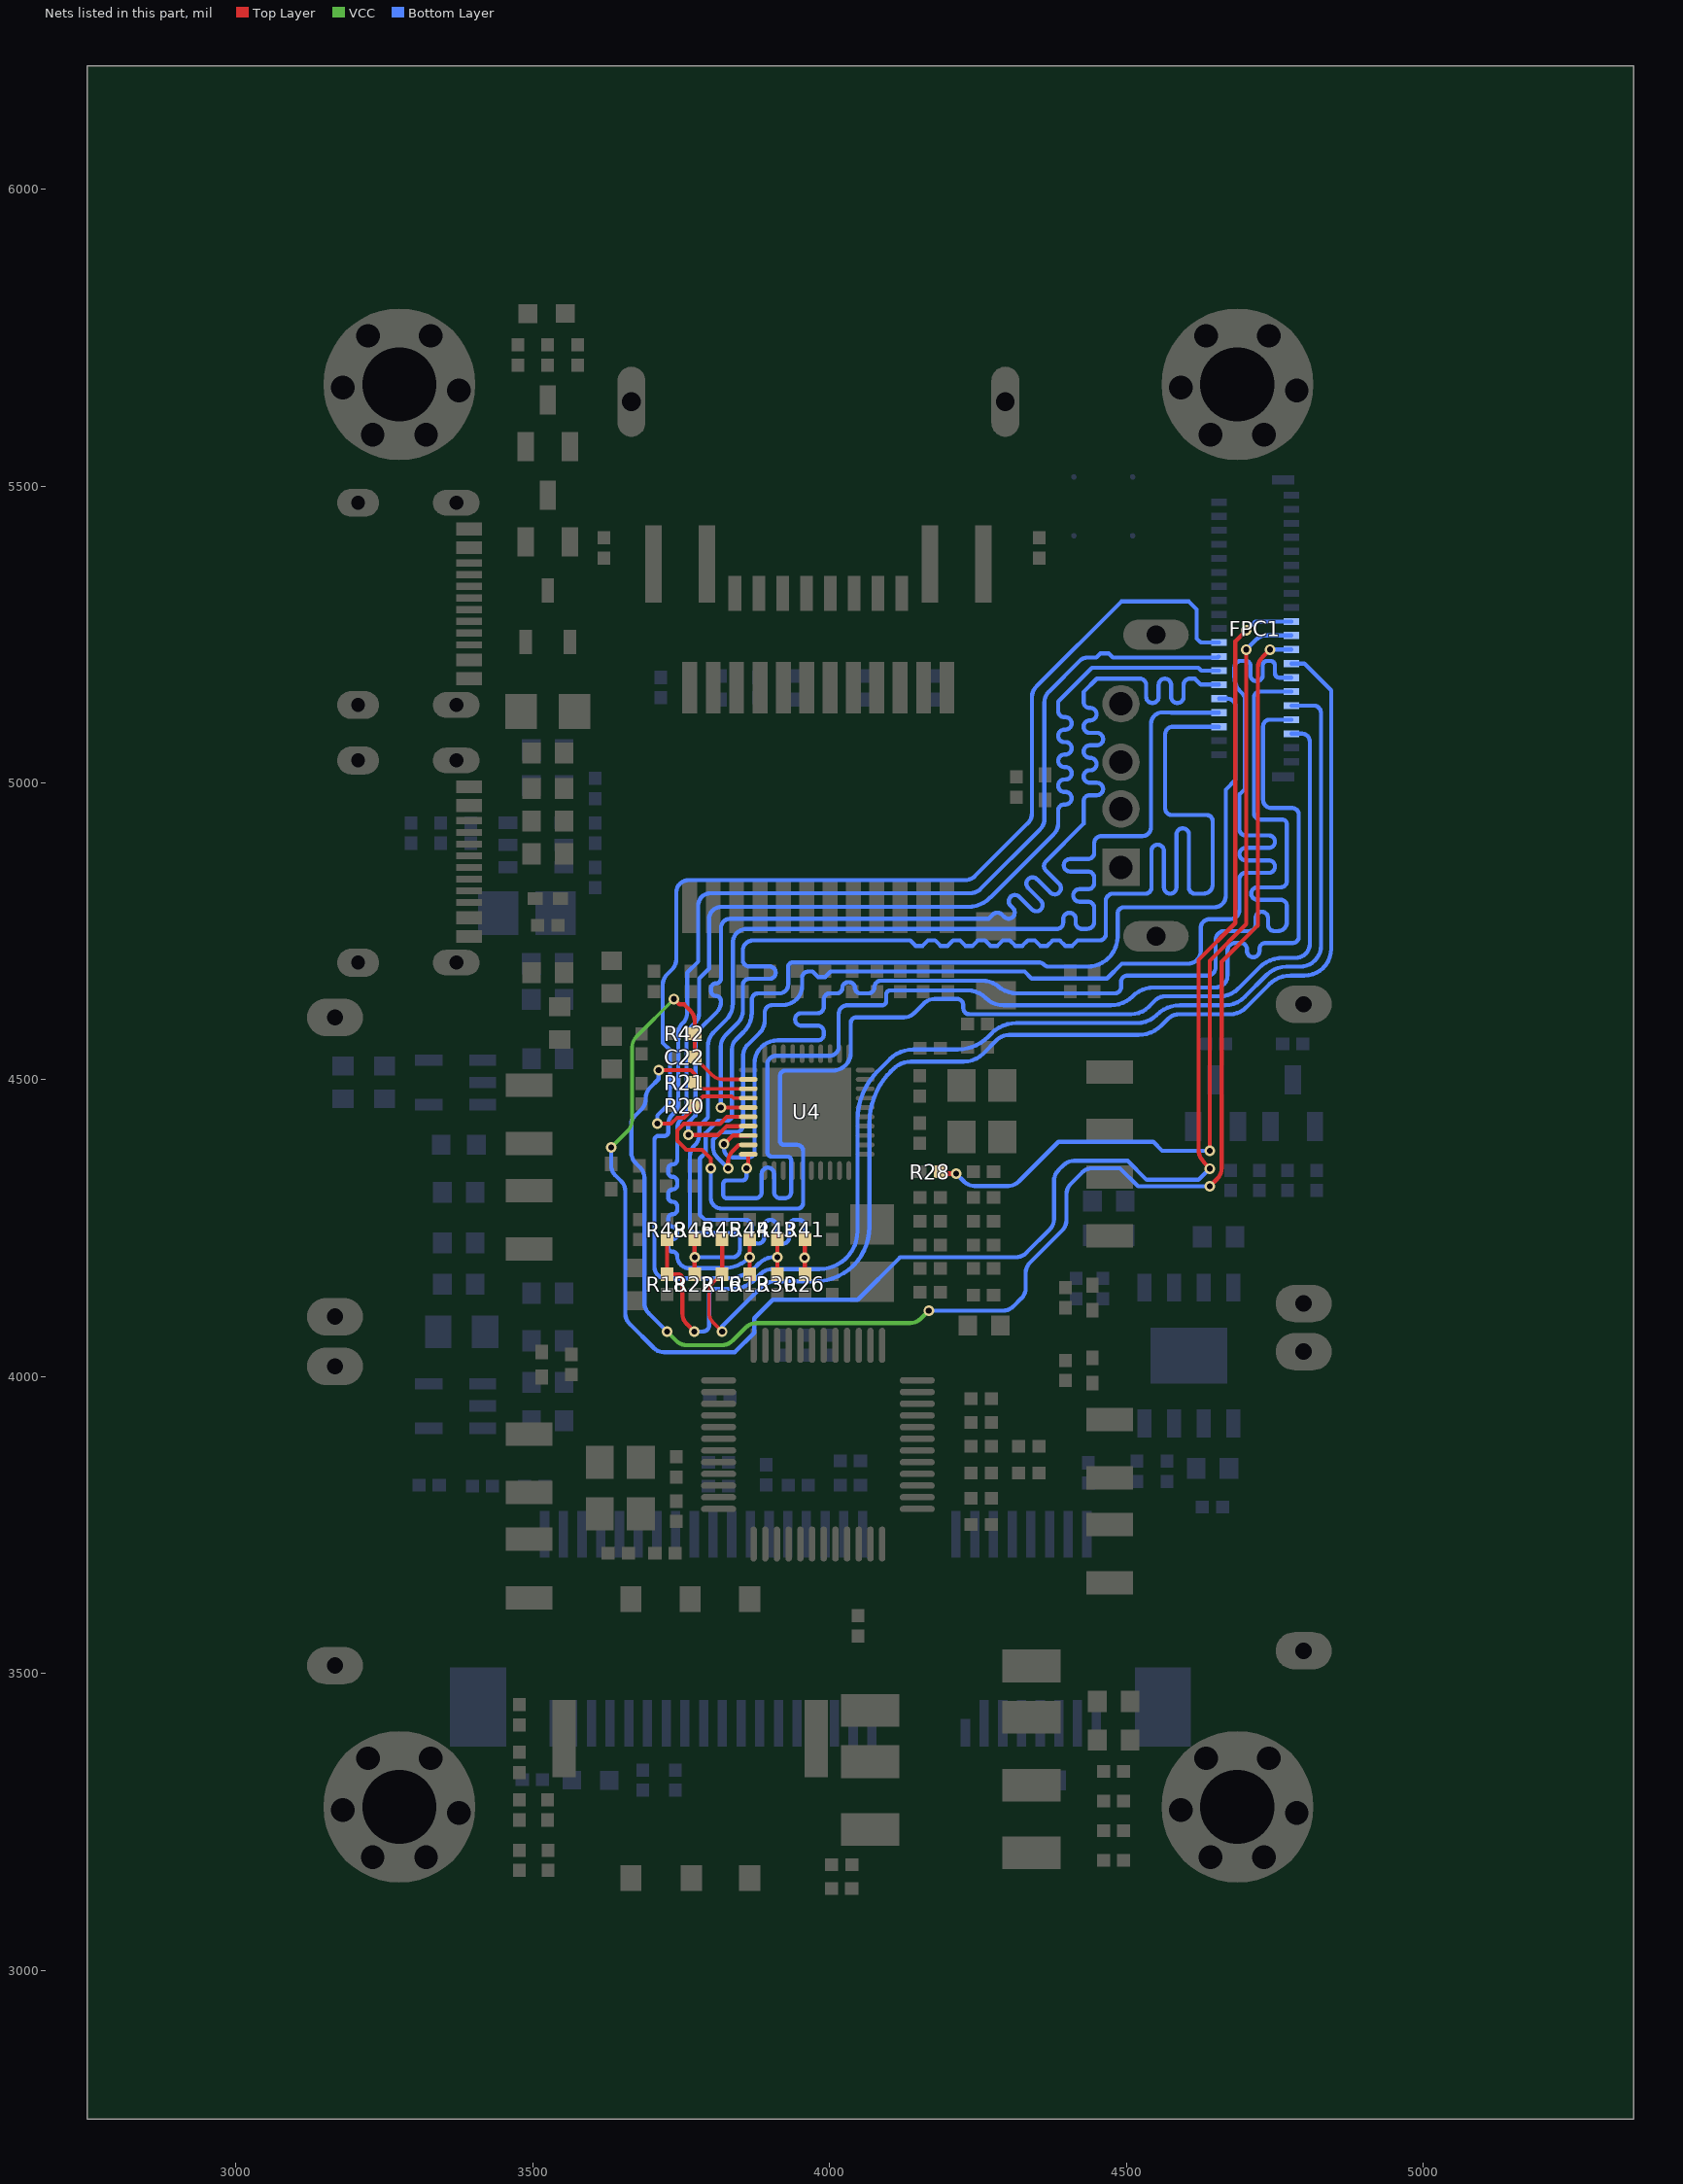
[diagram p0: the nets of this part, all layers, seen from the top]
# Altium PCB MISC84334.PcbDoc (part 5 of 8)
Units mil, origin at the board's own origin, x right, y up, seen from the top; angles counter-clockwise.
Board outline 2605.13 x 3457.4 mil, 4 copper layers (Top Layer, GND, VCC, Bottom Layer), stack 62.447 mil thick; 209 components, 149 nets, 735 pads, 529 vias.

## Via types
v1: diameter 18, hole 10, Top Layer to Bottom Layer, 529 vias

## Nets (pads, with @x,y where several pads share a name; then routed paths per layer and width w, separated by ;. In a path a pad name is that pad's centre, name@x,y a point inside that pad or via, vN(x,y) a via of type N, cw(c..) or ccw(c..) an arc to the next point about the centre after c; other vN are vias at no path point) (continued)
GMAC0_MCLKINOUT: FPC1.19 R28.2 | length 1451.4
  Top Layer w7: v1(4640.59,4380.59) 4640.59,4700.59 4702.29,4762.29 v1(4702.29,5224.65)
  Top Layer w8: R28.2@4186.94,4342.09 v1(4213.29,4342.09)
  Bottom Layer w7: v1@4213.39,4342.09 4226.97,4328.51 ccw(c4244.65,4346.19) 4244.65,4321.19 4301.05,4321.19 ccw(c4301.05,4346.19) 4318.73,4328.51 4385.8,4395.59 4545.59,4395.59 4560.59,4380.59 v1(4640.59,4380.59) ; v1(4702.29,5224.65) 4718.6,5240.96 cw(c4736.28,5223.28) 4736.28,5248.28 FPC1.19@4778.31,5248.27
GMAC0_MDC: FPC1.17 R21.2 U4.13 | length 2745
  Top Layer w6: R21.2@3773.13,4495.59 3783.73,4484.99 U4.13@3863.36,4484.99
  Top Layer w7: v1(3712.29,4516.19) 3766.66,4516.19 3773.13,4509.72 R21.2@3773.13,4495.59 ; v1(4640.59,4320.59) 4653.47,4333.47 ccw(c4635.79,4351.15) 4660.79,4351.15 4660.79,4698.96 4721.83,4760 4721.83,5193.84 cw(c4746.83,5193.84) 4729.16,5211.52 v1(4742.29,5224.65)
  VCC w7: v1(3726.29,4076.19) 3741.97,4060.51 ccw(c3759.65,4078.19) 3759.65,4053.19 3818.94,4053.19 ccw(c3818.94,4078.19) 3836.61,4060.51 3859.12,4083.02 cw(c3876.8,4065.34) 3876.8,4090.34 4136.09,4090.34 ccw(c4136.09,4115.34) 4153.77,4097.67 v1(4167.29,4111.19)
  Bottom Layer w7: 3689.29,4145.19 3688.29,4146.19 ; v1(3712.29,4516.19) 3712.29,4501.19 3697.91,4486.81 ccw(c3715.59,4469.14) 3690.59,4469.14 3690.59,4467.71 cw(c3665.59,4467.71) 3683.27,4450.03 3670.34,4437.1 ccw(c3680.1,4427.33) 3666.29,4427.33 3666.29,4377.55 ccw(c3691.29,4377.55) 3673.61,4359.87 3680.97,4352.51 cw(c3663.29,4334.84) 3688.29,4334.84 3688.29,4146.19 ; v1(3726.29,4076.19) 3695.61,4106.87 cw(c3713.29,4124.55) 3688.29,4124.55 3688.29,4146.19 ; v1(4167.29,4111.19) 4292.2,4111.19 ccw(c4292.2,4136.19) 4309.88,4118.51 4323.38,4132.02 ccw(c4305.71,4149.7) 4330.71,4149.7 4330.71,4174.5 cw(c4355.71,4174.5) 4338.03,4192.18 4391.97,4246.12 ccw(c4374.29,4263.8) 4399.29,4263.8 4399.29,4307.16 cw(c4424.29,4307.16) 4406.61,4324.84 4425.65,4343.87 cw(c4443.32,4326.19) 4443.32,4351.19 4489.45,4351.19 4520.05,4320.59 v1(4640.59,4320.59) ; v1(4742.29,5224.65) FPC1.17@4778.31,5224.65
GMAC0_MDIO: FPC1.18 R20.2 U4.14 | length 1887.1
  Top Layer w6: v1(3710.29,4426.19) 3733.29,4426.19 3743.29,4436.19 3755.29,4436.19 3773.13,4454.03 R20.2@3773.13,4456.33 3773.13,4458.16 3787.03,4472.05 3835.63,4472.05 3838.49,4469.19 U4.14@3863.36,4469.19
  Bottom Layer w7: v1@3711.29,4426.19 v1(3710.29,4426.19) 3710.29,4439.99 3723.97,4453.67 ccw(c3706.29,4471.34) 3731.29,4471.34 3731.29,4550.19 3719.29,4562.19 3719.29,4659.84 cw(c3744.29,4659.84) 3726.61,4677.51 3734.72,4685.62 ccw(c3717.05,4703.3) 3742.05,4703.3 3742.05,4815.59 cw(c3762.65,4815.59) 3762.65,4836.19 4227.94,4836.19 ccw(c4227.94,4861.19) 4245.61,4843.51 4333.97,4931.87 ccw(c4316.29,4949.55) 4341.29,4949.55 4341.29,5144.84 cw(c4366.29,5144.84) 4348.61,5162.51 4491.69,5305.59 4605.59,5305.59 4618.84,5292.34 4618.84,5243.21 4625.59,5236.46 FPC1.18@4656.27,5236.46
GMAC0_RSTN: C22.2 FPC1.21 R42.1 U4.12 | length 3058.2
  Top Layer w6: R42.1@3773.13,4578.09 C22.2@3773.13,4538.09 3773.13,4537.35 3802.47,4508.01 ccw(c3820.15,4525.69) 3820.15,4500.69 U4.12@3863.36,4500.69
  Top Layer w7: v1(3738.29,4636.19) 3747.39,4627.09 3755.39,4627.09 3765.81,4616.67 cw(c3748.13,4599) 3773.13,4599 R42.1@3773.13,4578.09 ; v1(4640.59,4350.59) 4628.53,4364.26 cw(c4647.86,4381.31) 4622.09,4381.31 4622.09,4702.09 4683.79,4763.79 4683.79,5238.4 v1(4702.29,5256.9)
  VCC w6: v1(3632.29,4386.19) 3660.27,4414.17 ccw(c3642.59,4431.85) 3667.59,4431.85 3667.59,4555.14 cw(c3692.59,4555.14) 3674.91,4572.81 v1(3738.29,4636.19)
  Bottom Layer w7: v1(3632.29,4386.19) 3632.29,4356.55 ccw(c3657.29,4356.55) 3639.61,4338.87 3648.97,4329.51 cw(c3631.29,4311.84) 3656.29,4311.84 3656.29,4106.55 ccw(c3681.29,4106.55) 3663.61,4088.87 3703.97,4048.51 ccw(c3721.65,4066.19) 3721.65,4041.19 3840.58,4041.19 3873.48,4074.09 3873.48,4098.6 3904.57,4129.69 4047.7,4129.69 4119.2,4201.19 4313.94,4201.19 ccw(c4313.94,4226.19) 4331.61,4208.51 4370.97,4247.87 ccw(c4353.29,4265.55) 4378.29,4265.55 4378.29,4329.81 cw(c4403.29,4329.81) 4385.61,4347.49 4394.49,4356.37 cw(c4412.17,4338.69) 4412.17,4363.69 4502.49,4363.69 4534.59,4331.59 4621.59,4331.59 v1(4640.59,4350.59) ; v1(4702.29,5256.9) 4717.29,5271.9 FPC1.21@4778.31,5271.89
GMAC0_RXCLK: FPC1.10 R26.2 R41.2 | length 2122.7
  Top Layer w7: R26.2@3958.66,4172.63 R41.2@3958.66,4230.81
  Bottom Layer w7: v1(3958.29,4200.19) 3958.29,4255.19 ccw(c3949.29,4255.19) 3949.29,4264.19 3942.71,4264.19 ccw(c3942.71,4253.69) 3932.21,4253.69 3932.21,4234.59 cw(c3921.71,4234.59) 3911.21,4234.59 3911.21,4253.69 ccw(c3900.71,4253.69) 3890.21,4253.69 3890.21,4234.59 cw(c3879.71,4234.59) 3869.21,4234.59 3869.21,4253.69 ccw(c3858.71,4253.69) 3858.71,4264.19 3790.29,4264.19 3781.8,4272.68 3781.8,4367.85 3791.79,4377.84 3791.79,4410.71 3812.29,4431.19 3827.29,4431.19 ccw(c3827.29,4439.69) 3835.79,4439.69 3835.79,4551.48 cw(c3858.27,4551.48) 3842.37,4567.37 3855.59,4580.59 ccw(c3822.52,4613.67) 3869.29,4613.67 3869.29,4635.08 cw(c3879.8,4635.08) 3879.8,4645.59 3915.59,4645.59 ccw(c3915.59,4660.59) 3930.59,4660.59 3930.59,4690.47 cw(c3937.81,4690.47) 3937.81,4697.69 4352.74,4697.69 cw(c4352.74,4685.57) 4361.31,4694.14 ccw(c4369.88,4702.71) 4369.88,4690.59 4434.44,4690.59 ccw(c4434.44,4741.65) 4470.55,4705.55 ccw(c4434.44,4741.65) 4485.5,4741.65 4485.5,4779.75 cw(c4496.34,4779.75) 4496.34,4790.59 4648.37,4790.59 ccw(c4648.37,4809.87) 4667.65,4809.87 4667.65,4988.76 4684.29,5005.4 4684.29,5127.96 ccw(c4670.27,5127.96) 4680.18,5137.87 ccw(c4670.27,5127.96) 4670.27,5141.98 FPC1.10@4656.27,5141.97
GMAC0_RXD0: FPC1.14 R13.2 R44.2 | length 2125.2
  Top Layer w7: R13.2@3865.8,4172.63 v1(3865.8,4201.17) R44.2@3865.8,4230.81
  Bottom Layer w7: v1(3865.8,4201.17) cw(c3821.19,4245.79) 3821.19,4182.69 3763.93,4182.69 cw(c3763.93,4203.03) 3743.59,4203.03 ccw(c3735.99,4203.03) 3735.99,4210.63 cw(c3735.99,4218.23) 3728.39,4218.23 3728.39,4224.03 cw(c3735.99,4224.03) 3735.99,4231.63 ccw(c3735.99,4239.23) 3743.59,4239.23 3743.59,4245.03 ccw(c3735.99,4245.03) 3735.99,4252.63 cw(c3735.99,4260.23) 3728.39,4260.23 3728.39,4266.03 cw(c3735.99,4266.03) 3735.99,4273.63 ccw(c3735.99,4281.23) 3743.59,4281.23 3743.59,4287.03 ccw(c3735.99,4287.03) 3735.99,4294.63 cw(c3735.99,4302.23) 3728.39,4302.23 3728.39,4308.03 cw(c3735.99,4308.03) 3735.99,4315.63 ccw(c3735.99,4323.23) 3743.59,4323.23 3743.59,4329.03 ccw(c3735.99,4329.03) 3735.99,4336.63 cw(c3735.99,4344.23) 3728.39,4344.23 3728.39,4350.03 cw(c3735.99,4350.03) 3735.99,4357.63 ccw(c3735.99,4365.23) 3743.59,4365.23 3743.59,4417.14 cw(c3768.59,4417.14) 3750.91,4434.81 3751.97,4435.87 ccw(c3734.29,4453.55) 3759.29,4453.55 3759.29,4571.08 cw(c3784.29,4571.08) 3766.61,4588.76 3773.29,4595.44 ccw(c3755.68,4613.06) 3780.59,4613.06 3780.59,4670.59 3797.29,4687.29 3797.29,4770.84 cw(c3817.65,4770.84) 3817.65,4791.19 4232.9,4791.19 ccw(c4232.9,4845.33) 4271.18,4807.05 4377.97,4913.84 ccw(c4360.29,4931.51) 4385.29,4931.51 4385.29,4953.33 cw(c4395.79,4953.33) 4395.79,4963.83 4397.61,4963.83 ccw(c4397.61,4974.33) 4397.61,4984.83 4395.79,4984.83 cw(c4395.79,4995.33) 4395.79,5005.83 4397.61,5005.83 ccw(c4397.61,5016.33) 4397.61,5026.83 4395.79,5026.83 cw(c4395.79,5037.33) 4395.79,5047.83 4397.61,5047.83 ccw(c4397.61,5058.33) 4397.61,5068.83 4395.79,5068.83 cw(c4395.79,5079.33) 4395.79,5089.83 4397.61,5089.83 ccw(c4397.61,5100.33) 4397.61,5110.83 4395.79,5110.83 cw(c4395.79,5121.33) 4385.29,5121.33 4385.29,5137.19 4442.24,5194.14 4621.44,5194.14 4626.36,5189.22 FPC1.14@4656.27,5189.22
GMAC0_RXD1: FPC1.15 R16.2 R45.2 | length 2125.3
  Top Layer w6: v1(3819.38,4076.19) 3804.61,4090.95 cw(c3822.29,4108.63) 3797.29,4108.63 3797.29,4141.59 cw(c3822.29,4141.59) 3804.61,4159.27 3817.98,4172.63 R16.2@3819.38,4172.63
  Top Layer w7: R16.2@3819.38,4172.63 R45.2@3819.38,4230.81
  Bottom Layer w7: v1(3819.38,4076.19) 3819.38,4085.03 3885.76,4151.41 cw(c3907.92,4129.26) 3907.92,4160.59 3975.88,4160.59 ccw(c3975.88,4252.01) 4067.29,4252.01 4067.29,4426.65 cw(c4192.12,4426.65) 4097.07,4507.56 4102.78,4513.28 cw(c4118.29,4503.19) 4108.2,4518.7 cw(c4136.91,4489.98) 4115.77,4524.65 cw(c4136.91,4489.98) 4136.91,4530.59 4226.3,4530.59 ccw(c4226.3,4577.16) 4259.23,4544.23 4282.44,4567.44 cw(c4302.12,4547.75) 4302.12,4575.59 4520.6,4575.59 ccw(c4520.6,4630.46) 4559.4,4591.66 4570.54,4602.8 cw(c4589.35,4583.98) 4589.35,4610.59 4675.41,4610.59 ccw(c4675.41,4647.24) 4701.32,4621.32 4740.59,4660.59 cw(c4776.8,4624.38) 4776.8,4675.59 4800.09,4675.59 ccw(c4800.09,4720.78) 4845.28,4720.78 4845.28,5155.9 4800.15,5201.03 FPC1.15@4778.31,5201.03
GMAC0_RXD2: FPC1.8 R22.2 R46.2 | length 2122.7
  Top Layer w7: R22.2@3772.95,4172.63 R46.2@3772.95,4230.81
  Bottom Layer w7: v1(3773.29,4201.19) 3836.29,4201.19 ccw(c3836.29,4214.19) 3849.29,4214.19 3849.29,4234.18 ccw(c3841.28,4234.18) 3841.28,4242.19 3775.16,4242.19 cw(c3775.16,4252.42) 3764.93,4252.42 3764.93,4371.25 cw(c3789.93,4371.25) 3772.25,4388.93 3773.47,4390.14 ccw(c3755.79,4407.82) 3780.79,4407.82 3780.79,4421.95 3795.29,4436.45 3795.29,4556.63 cw(c3828.26,4556.63) 3804.95,4579.95 3825.59,4600.59 ccw(c3797.34,4628.84) 3837.29,4628.84 3837.29,4730.84 cw(c3860.65,4730.84) 3860.65,4754.19 4383.37,4754.19 ccw(c4383.37,4764.69) 4393.87,4764.69 4393.87,4770.86 cw(c4404.37,4770.86) 4414.87,4770.86 4414.87,4764.69 ccw(c4425.37,4764.69) 4425.37,4754.19 4434.19,4754.19 ccw(c4434.19,4766.09) 4446.09,4766.09 4446.09,4789.54 ccw(c4435.59,4789.54) 4435.59,4800.04 4421.09,4800.04 cw(c4421.09,4810.54) 4421.09,4821.04 4435.59,4821.04 ccw(c4435.59,4831.54) 4446.09,4831.54 4446.09,4840.38 ccw(c4435.59,4840.38) 4435.59,4850.88 4405.29,4850.88 cw(c4405.29,4861.38) 4405.29,4871.88 4435.59,4871.88 ccw(c4435.59,4882.38) 4446.09,4882.38 4446.09,4898.59 cw(c4458.09,4898.59) 4458.09,4910.59 4527.28,4910.59 ccw(c4527.28,4925.01) 4541.7,4925.01 4541.7,5099.48 cw(c4561.02,5099.48) 4561.02,5118.8 4592.83,5118.35 ; 4575.62,5118.35 4592.84,5118.35 ; FPC1.8@4656.27,5118.35 4592.84,5118.35
GMAC0_RXD3: FPC1.9 R18.2 R48.2 | length 2120
  Top Layer w7: R48.2@3726.52,4230.81 R18.2@3726.52,4172.63 3744.8,4172.63 cw(c3744.8,4165.14) 3752.29,4165.14 3752.29,4106.55 ccw(c3777.29,4106.55) 3759.61,4088.87 v1(3772.29,4076.19)
  Bottom Layer w7: v1(3772.29,4076.19) 3787.29,4076.19 ccw(c3787.29,4086.19) 3797.29,4086.19 3797.29,4137.79 cw(c3807.59,4137.79) 3807.59,4148.09 3835.59,4148.09 ccw(c3835.59,4205.07) 3875.88,4164.78 3884.97,4173.87 cw(c3902.65,4156.19) 3902.65,4181.19 3983.06,4181.19 ccw(c3983.06,4245.42) 4013.57,4188.9 ccw(c3983.06,4245.42) 4047.29,4245.42 4047.29,4432.02 cw(c4164.38,4432.02) 4081.59,4514.82 4101.28,4534.51 cw(c4141.55,4494.25) 4141.55,4551.19 4216.09,4551.19 ccw(c4216.09,4623.86) 4267.48,4572.48 4273.62,4578.62 cw(c4314.59,4537.65) 4314.59,4595.59 4517.91,4595.59 ccw(c4517.91,4643.17) 4551.56,4609.53 cw(c4590.34,4570.75) 4590.34,4625.59 4666.52,4625.59 ccw(c4666.52,4671.64) 4699.08,4639.08 4737.04,4677.04 cw(c4769.75,4644.33) 4769.75,4690.59 4792.99,4690.59 ccw(c4792.99,4725.68) 4828.08,4725.68 4828.08,5118.14 ccw(c4816.05,5118.14) 4816.05,5130.17 FPC1.9@4778.31,5130.16
GMAC0_RXDV_CRS: FPC1.16 R30.2 R43.2 | length 2122.3
  Top Layer w7: R30.2@3912.23,4172.63 v1(3912.23,4201.17) R43.2@3912.23,4230.81
  Bottom Layer w7: FPC1.16@4656.27,5212.84 cw(c4652.21,5216.9) 4652.21,5211.16 4477.56,5211.16 4470.56,5218.16 4456.56,5218.16 4449.56,5211.16 4434.14,5211.16 ccw(c4434.14,5194.55) 4422.39,5206.29 4369.61,5153.51 ccw(c4387.29,5135.84) 4362.29,5135.84 4362.29,4939.55 cw(c4337.29,4939.55) 4354.97,4921.87 4254.61,4821.51 cw(c4236.94,4839.19) 4236.94,4814.19 3799.34,4814.19 ccw(c3799.34,4793.9) 3779.05,4793.9 3779.05,4699.05 3760.59,4680.59 3760.59,4614.34 cw(c3733.35,4614.34) 3752.61,4595.09 ccw(c3770.29,4577.41) 3745.29,4577.41 3745.29,4461.55 cw(c3720.29,4461.55) 3737.97,4443.87 3734.36,4440.26 ccw(c3747.83,4426.79) 3728.78,4426.79 cw(c3710.29,4426.19) 3728.78,4425.59 3728.78,4412.41 cw(c3721.96,4412.41) 3721.96,4405.59 3712.37,4405.59 ccw(c3712.37,4398.52) 3705.29,4398.52 3705.29,4184.68 ccw(c3724.41,4184.68) 3724.41,4165.55 3826.26,4165.55 ccw(c3826.26,4238.19) 3849.97,4169.53 ccw(c3826.26,4238.19) 3854.79,4171.39 ccw(c3826.26,4238.19) 3877.62,4186.83 3881.75,4190.95 cw(c3907.26,4165.44) 3902.28,4201.17 ; 3902.28,4201.17 v1(3912.23,4201.17) ccw(c3907.26,4165.44) 3902.28,4201.17
GMAC0_TXCLK: FPC1.7 U4.20 | length 2125.1
  Top Layer w7: v1(3860.4,4351.11) 3863.36,4354.07 U4.20@3863.36,4374.69
  Bottom Layer w7: v1(3860.4,4351.11) 3860.4,4337.84 cw(c3853.14,4337.84) 3853.14,4330.59 3827,4330.59 ccw(c3827,4324.77) 3821.17,4324.77 3821.17,4306.93 ccw(c3827.51,4306.93) 3827.51,4300.59 3875.4,4300.59 ccw(c3875.4,4311.09) 3885.9,4311.09 3885.9,4341.61 cw(c3896.4,4341.61) 3906.9,4341.61 3906.9,4311.09 ccw(c3917.4,4311.09) 3917.4,4300.59 3924.98,4300.59 ccw(c3924.98,4311.2) 3935.59,4311.2 3935.59,4364.53 ccw(c3929.53,4364.53) 3929.53,4370.59 3903.44,4370.59 cw(c3903.44,4378.52) 3895.52,4378.52 3895.52,4525.98 cw(c3910.13,4525.98) 3910.13,4540.59 4000.59,4540.59 ccw(c4000.59,4555.59) 4015.59,4555.59 4015.59,4610.59 cw(c4030.59,4610.59) 4030.59,4625.59 4088.81,4625.59 ccw(c4088.81,4632.37) 4095.59,4632.37 4095.59,4643.95 cw(c4102.23,4643.95) 4102.23,4650.59 4232.91,4650.59 cw(c4232.91,4607.91) 4263.09,4638.09 ccw(c4293.27,4668.27) 4293.27,4625.59 4474.38,4625.59 ccw(c4474.38,4676.8) 4510.59,4640.59 cw(c4546.8,4604.38) 4546.8,4655.59 4650.59,4655.59 ccw(c4650.59,4675.59) 4670.59,4675.59 4670.59,4717.64 cw(c4683.54,4717.64) 4683.54,4730.59 4692.93,4730.59 cw(c4692.93,4720.09) 4703.43,4720.09 4703.43,4716.99 ccw(c4713.93,4716.99) 4724.43,4716.99 4724.43,4720.09 cw(c4734.93,4720.09) 4734.93,4730.59 4780.59,4730.59 ccw(c4780.59,4740.59) 4790.59,4740.59 4790.59,4947.03 ccw(c4779.93,4947.03) 4779.93,4957.69 4744.71,4957.69 cw(c4744.71,4971.81) 4730.59,4971.81 4730.59,5095.59 cw(c4741.54,5095.59) 4741.54,5106.54 FPC1.7@4778.31,5106.54
GMAC0_TXD0: FPC1.11 U4.18 | length 2120.8
  Top Layer w7: v1(3822.34,4391.63) 3822.73,4391.63 3837.29,4406.19 U4.18@3863.36,4406.19
  Bottom Layer w7: v1(3822.34,4391.63) 3822.34,4383.84 ccw(c3836.57,4383.84) 3836.57,4369.61 3864.61,4369.61 ccw(c3864.61,4378.82) 3873.82,4378.82 3873.82,4527.51 cw(c3912.87,4527.51) 3912.87,4566.55 3980.65,4566.55 ccw(c3980.65,4576.49) 3990.59,4576.49 3990.59,4580.7 ccw(c3980.09,4580.7) 3980.09,4591.2 3952.75,4591.2 cw(c3952.75,4601.7) 3952.75,4612.2 3980.09,4612.2 ccw(c3980.09,4622.7) 3990.59,4622.7 3990.59,4635.59 cw(c4000.59,4635.59) 4000.59,4645.59 4012.54,4645.59 ccw(c4012.54,4654.96) 4021.91,4654.96 cw(c4031.29,4654.96) 4031.29,4664.33 4033.54,4664.33 cw(c4033.54,4654.96) 4042.91,4654.96 ccw(c4052.29,4654.96) 4052.29,4645.59 4065.59,4645.59 ccw(c4065.59,4655.59) 4075.59,4655.59 cw(c4087.05,4655.59) 4087.05,4667.05 4257.06,4667.05 cw(c4257.06,4622.04) 4281.08,4660.1 ; FPC1.11@4778.31,5153.78 4725.11,5153.79 ccw(c4725.11,5143.97) 4715.29,5143.97 4715.29,4949.2 ccw(c4726.08,4949.2) 4726.08,4938.41 4762.77,4938.41 cw(c4762.77,4930.59) 4770.59,4930.59 4770.59,4834.73 cw(c4760.09,4834.73) 4760.09,4824.23 4721.09,4824.23 ccw(c4721.09,4813.73) 4721.09,4803.23 4760.09,4803.23 cw(c4760.09,4792.73) 4770.59,4792.73 4770.59,4765.59 cw(c4755.59,4765.59) 4755.59,4750.59 4749.38,4750.59 cw(c4749.38,4761.09) 4738.88,4761.09 4738.88,4772.64 ccw(c4728.38,4772.64) 4717.88,4772.64 4717.88,4761.09 cw(c4707.38,4761.09) 4707.38,4750.59 4665.59,4750.59 ccw(c4665.59,4735.59) 4650.59,4735.59 4650.59,4689.39 cw(c4636.79,4689.39) 4636.79,4675.59 4501.9,4675.59 ccw(c4501.9,4665.16) 4491.47,4665.16 4491.47,4656.47 cw(c4480.59,4656.47) 4480.59,4645.59 4316.8,4645.59 cw(c4316.8,4696.8) 4288.89,4653.87 ; 4281.08,4660.1 cw(c4257.06,4622.04) 4288.89,4653.87 ; 4281.08,4660.1 ccw(c4316.8,4696.8) 4288.89,4653.87
GMAC0_TXD1: FPC1.12 U4.17 | length 2126.1
  Top Layer w7: v1(3762.29,4407.19) 3812.34,4407.19 3827.14,4421.99 U4.17@3863.36,4421.99
  Bottom Layer w7: v1(3762.29,4407.19) 3762.29,4427.99 3774.29,4439.99 3774.29,4567.84 cw(c3799.29,4567.84) 3781.61,4585.51 3809.97,4613.87 ccw(c3792.29,4631.55) 3817.29,4631.55 3817.29,4632.94 ccw(c3808.89,4632.94) 3808.89,4641.34 cw(c3808.89,4649.74) 3800.49,4649.74 3800.49,4653.94 cw(c3808.89,4653.94) 3808.89,4662.34 ccw(c3808.89,4670.74) 3817.29,4670.74 3817.29,4755.84 cw(c3832.65,4755.84) 3832.65,4771.19 4268.18,4771.19 4275.46,4778.47 cw(c4282.88,4771.04) 4290.31,4778.47 4294.29,4774.48 ccw(c4301.72,4781.91) 4309.14,4789.33 4305.16,4793.32 cw(c4312.58,4800.74) 4320.01,4808.17 4341.22,4786.95 ccw(c4348.65,4794.38) 4356.07,4801.8 4334.85,4823.02 cw(c4342.28,4830.44) 4349.7,4837.87 4372.11,4815.46 ccw(c4379.53,4822.88) 4386.96,4830.31 4364.55,4852.71 cw(c4371.98,4860.14) 4364.55,4867.56 4428.17,4931.18 4428.17,4968.84 cw(c4438.67,4968.84) 4438.67,4979.34 4450.52,4979.34 ccw(c4450.52,4989.84) 4450.52,5000.34 4438.67,5000.34 cw(c4438.67,5010.84) 4438.67,5021.34 4439.56,5021.34 ccw(c4439.56,5031.84) 4439.56,5042.34 4438.67,5042.34 cw(c4438.67,5052.84) 4438.67,5063.34 4450.52,5063.34 ccw(c4450.52,5073.84) 4450.52,5084.34 4438.67,5084.34 cw(c4438.67,5094.84) 4438.67,5105.34 4439.56,5105.34 ccw(c4439.56,5115.84) 4439.56,5126.34 4438.67,5126.34 cw(c4438.67,5136.84) 4428.17,5136.84 4428.17,5153.17 4450.59,5175.59 4523.13,5175.59 cw(c4523.13,5165.09) 4533.63,5165.09 4533.63,5145.17 ccw(c4544.13,5145.17) 4554.63,5145.17 4554.63,5165.09 cw(c4565.13,5165.09) 4575.63,5165.09 4575.63,5145.17 ccw(c4586.13,5145.17) 4596.63,5145.17 4596.63,5165.09 cw(c4607.13,5165.09) 4607.13,5175.59 4615.59,5175.59 4625.58,5165.6 FPC1.12@4656.27,5165.6
GMAC0_TXD2: FPC1.5 U4.16 | length 2120.8
  Top Layer w7: v1(3800.3,4351.11) 3800.3,4367.47 3785.66,4382.11 3759.1,4382.11 3743.79,4397.42 3743.79,4414.85 3754.63,4425.69 3815.28,4425.69 3827.28,4437.69 U4.16@3863.36,4437.69
  Bottom Layer w7: v1(3800.3,4351.11) 3800.3,4300.88 ccw(c3818.05,4300.88) 3818.05,4283.13 3946.49,4283.13 ccw(c3946.49,4292.23) 3955.59,4292.23 3955.59,4380.59 ccw(c3945.59,4380.59) 3945.59,4390.59 3923.43,4390.59 cw(c3923.43,4397.28) 3916.74,4397.28 3916.74,4506.25 cw(c3926.08,4506.25) 3926.08,4515.59 4005.59,4515.59 ccw(c4005.59,4546.11) 4036.11,4546.11 4036.11,4596.11 cw(c4045.19,4596.11) 4045.19,4605.19 4125.28,4605.19 ccw(c4125.28,4630.19) 4142.95,4612.51 4159.31,4628.87 cw(c4176.99,4611.19) 4176.99,4636.19 4215.06,4636.19 cw(c4215.06,4625.66) 4225.59,4625.66 4225.59,4620.66 ; 4225.59,4620.59 ccw(c4235.59,4620.59) 4235.59,4610.59 4508.27,4610.59 ccw(c4508.27,4652.4) 4537.84,4622.84 4548.44,4633.44 cw(c4565.7,4616.19) 4565.7,4640.59 4657.74,4640.59 ccw(c4657.74,4683.69) 4688.21,4653.21 4723.31,4688.31 cw(c4765.03,4646.58) 4765.03,4705.59 4785.59,4705.59 ccw(c4785.59,4729.29) 4809.29,4729.29 4809.29,5069.76 ccw(c4796.13,5069.76) 4796.13,5082.92 FPC1.5@4778.31,5082.92
GMAC0_TXD3: FPC1.6 U4.15 | length 2118.5
  Top Layer w7: v1@3817.06,4453.49 U4.15@3863.36,4453.49
  Bottom Layer w7: v1(3817.03,4453.46) 3817.03,4555.58 cw(c3844.68,4555.58) 3825.13,4575.13 3845.59,4595.59 ccw(c3825.02,4616.16) 3854.11,4616.16 3854.11,4659.56 cw(c3864.61,4659.56) 3864.61,4670.06 3898.99,4670.06 ccw(c3898.99,4680.56) 3898.99,4691.06 3864.61,4691.06 cw(c3864.61,4701.56) 3854.11,4701.56 3854.11,4717.85 cw(c3870.95,4717.85) 3870.95,4734.69 4136.1,4734.69 4145.13,4725.66 4157.1,4725.66 4166.13,4734.69 4178.1,4734.69 4187.13,4725.66 4199.1,4725.66 4208.13,4734.69 4220.1,4734.69 4229.13,4725.66 4241.1,4725.66 4250.13,4734.69 4262.1,4734.69 4271.13,4725.66 4283.1,4725.66 4292.13,4734.69 4304.1,4734.69 4313.13,4725.66 4325.1,4725.66 4334.13,4734.69 4346.1,4734.69 4355.13,4725.66 4367.1,4725.66 4376.13,4734.69 4388.1,4734.69 4397.13,4725.66 4409.1,4725.66 4418.13,4734.69 4454.69,4734.69 ccw(c4454.69,4745.59) 4465.59,4745.59 4465.59,4801.1 cw(c4477.94,4801.1) 4477.94,4813.44 4532.06,4813.44 ccw(c4532.06,4823.94) 4542.56,4823.94 4542.56,4885.52 cw(c4553.06,4885.52) 4563.56,4885.52 4563.56,4823.94 ccw(c4574.06,4823.94) 4584.56,4823.94 4584.56,4913.07 cw(c4595.06,4913.07) 4605.56,4913.07 4605.56,4823.94 ccw(c4616.06,4823.94) 4616.06,4813.44 4630.29,4813.44 ccw(c4630.29,4828.75) 4645.59,4828.75 4645.59,4935.76 ccw(c4635.41,4935.76) 4635.41,4945.94 4576.93,4945.94 cw(c4576.93,4957.28) 4565.59,4957.28 4565.59,5081.68 cw(c4578.65,5081.68) 4578.65,5094.73 FPC1.6@4656.27,5094.73
GMAC0_TXEN: FPC1.13 U4.19 | length 2118.7
  Top Layer w7: v1(3829.34,4351.11) 3829.34,4362.11 cw(c3854.34,4362.11) 3836.66,4379.78 3847.37,4390.49 U4.19@3863.36,4390.49
  Bottom Layer w7: v1(3829.34,4351.11) 3811.16,4369.29 cw(c3828.84,4386.96) 3803.84,4386.96 3803.84,4399.29 3816.51,4411.96 3842.7,4411.96 ccw(c3842.7,4423.94) 3854.68,4423.94 3854.68,4540.74 cw(c3880.39,4540.74) 3854.75,4542.55 cw(c3880.39,4540.74) 3862.21,4558.92 3882.76,4579.47 ccw(c3862.92,4599.32) 3890.98,4599.32 3890.98,4613.1 cw(c3903.87,4613.1) 3903.87,4625.98 3921.34,4625.98 ccw(c3921.34,4658.67) 3954.03,4658.67 3954.03,4672.09 cw(c3964.28,4672.09) 3964.28,4682.34 3971.75,4682.34 3981.01,4673.07 3992.75,4673.07 4002.01,4682.34 4328.84,4682.34 4340.59,4670.59 4467.74,4670.59 4492.74,4695.59 4604.05,4695.59 ccw(c4604.05,4717.13) 4625.59,4717.13 4625.59,4755.59 cw(c4640.59,4755.59) 4640.59,4770.59 4674.93,4770.59 ccw(c4674.93,4786.25) 4690.59,4786.25 4690.59,4838.1 cw(c4701.09,4838.1) 4701.09,4848.6 4740.09,4848.6 ccw(c4740.09,4859.1) 4740.09,4869.6 4701.09,4869.6 cw(c4701.09,4880.1) 4701.09,4890.6 4740.09,4890.6 ccw(c4740.09,4901.1) 4740.09,4911.6 4701.09,4911.6 cw(c4701.09,4922.1) 4690.59,4922.1 4690.59,4980.59 4700.29,4990.29 4700.29,5139.24 ccw(c4684.24,5139.24) 4695.59,5150.59 4692.35,5153.83 cw(c4716.77,5178.26) 4682.61,5173.12 cw(c4716.77,5178.26) 4682.23,5178.26 4682.23,5194.47 cw(c4693.35,5194.47) 4693.35,5205.59 4701.02,5205.59 cw(c4701.02,5197.61) 4709,5197.61 4709,5181.99 ccw(c4719.5,5181.99) 4730,5181.99 4730,5198.54 cw(c4737.05,5198.54) 4737.05,5205.59 4742.64,5205.59 cw(c4742.64,5197.64) 4750.59,5197.64 4750.59,5184.35 ccw(c4757.53,5184.35) 4757.53,5177.41 FPC1.13@4778.31,5177.41